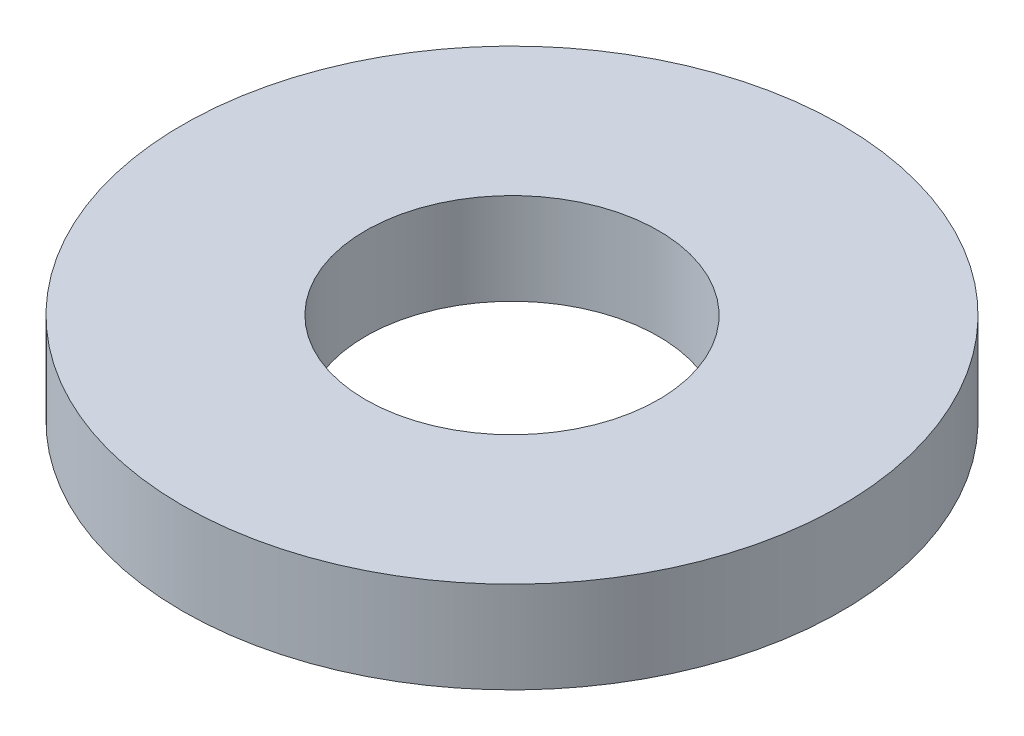
SolidWorks part; units mm, degrees
ref_plane "Front Plane" through (0, 0, 0) normal (0, 0, 1) x (1, 0, 0)
ref_plane "Top Plane" through (0, 0, 0) normal (0, 1, 0) x (1, 0, 0)
ref_plane "Right Plane" through (0, 0, 0) normal (1, 0, 0) x (0, 0, -1)
sketch "Sketch1" plane through (0, 0, 0) normal (0, 1, 0) x (1, 0, 0)
  circle A0 centre (0, 0) radius 8
  circle A1 centre (0, 0) radius 18
  dimension "D1" = 16
  dimension "D2" = 10
extrude "Boss-Extrude1" add sketch "Sketch1" along normal blind 5
